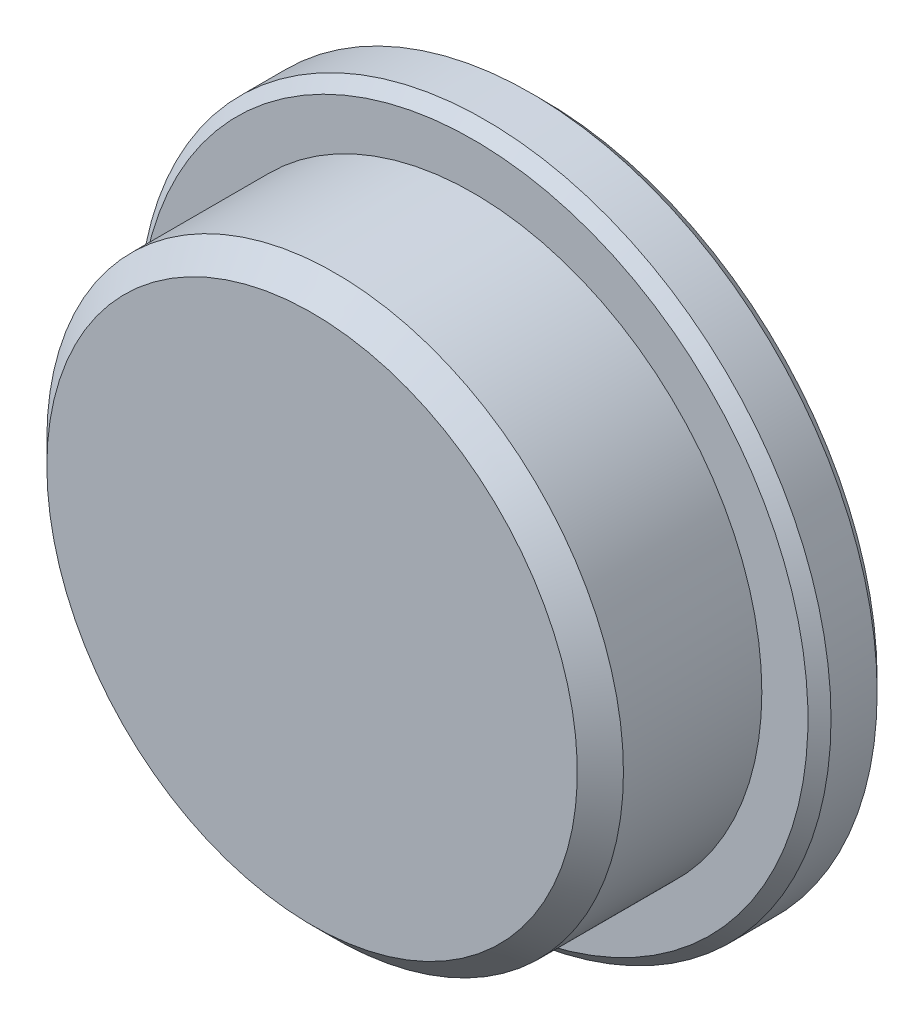
from build123d import *

# Parameters (mm, degrees)
CHAMFER1_SIZE = 1
CHAMFER2_SIZE = 0.5


with BuildPart() as part:
    # Sketch1 → Revolve1 (revolve)
    with BuildSketch(Plane(origin=(0, 0, 0), x_dir=(0, 0, -1), z_dir=(1, 0, 0)), mode=Mode.PRIVATE) as revolve1_sk:
        Polygon((10, 0), (10, 15), (7, 15), (7, 12.5), (0, 12.5), (0, 0), align=None)
    revolve(revolve1_sk.sketch.rotate(Axis((0, 0, 0), (0, 0, -1)), 90), axis=Axis((0, 0, 0), (0, 0, -1)))

    # Chamfer1
    chamfer1_edges = [part.edges().sort_by_distance(p)[0] for p in [
        (-12.5, 0, 0),
    ]]
    chamfer(chamfer1_edges, length=CHAMFER1_SIZE)

    # Chamfer2
    chamfer2_edges = [part.edges().sort_by_distance(p)[0] for p in [
        (-15, 0, -7),
        (-15, 0, -10),
    ]]
    chamfer(chamfer2_edges, length=CHAMFER2_SIZE)


solid = part.part
